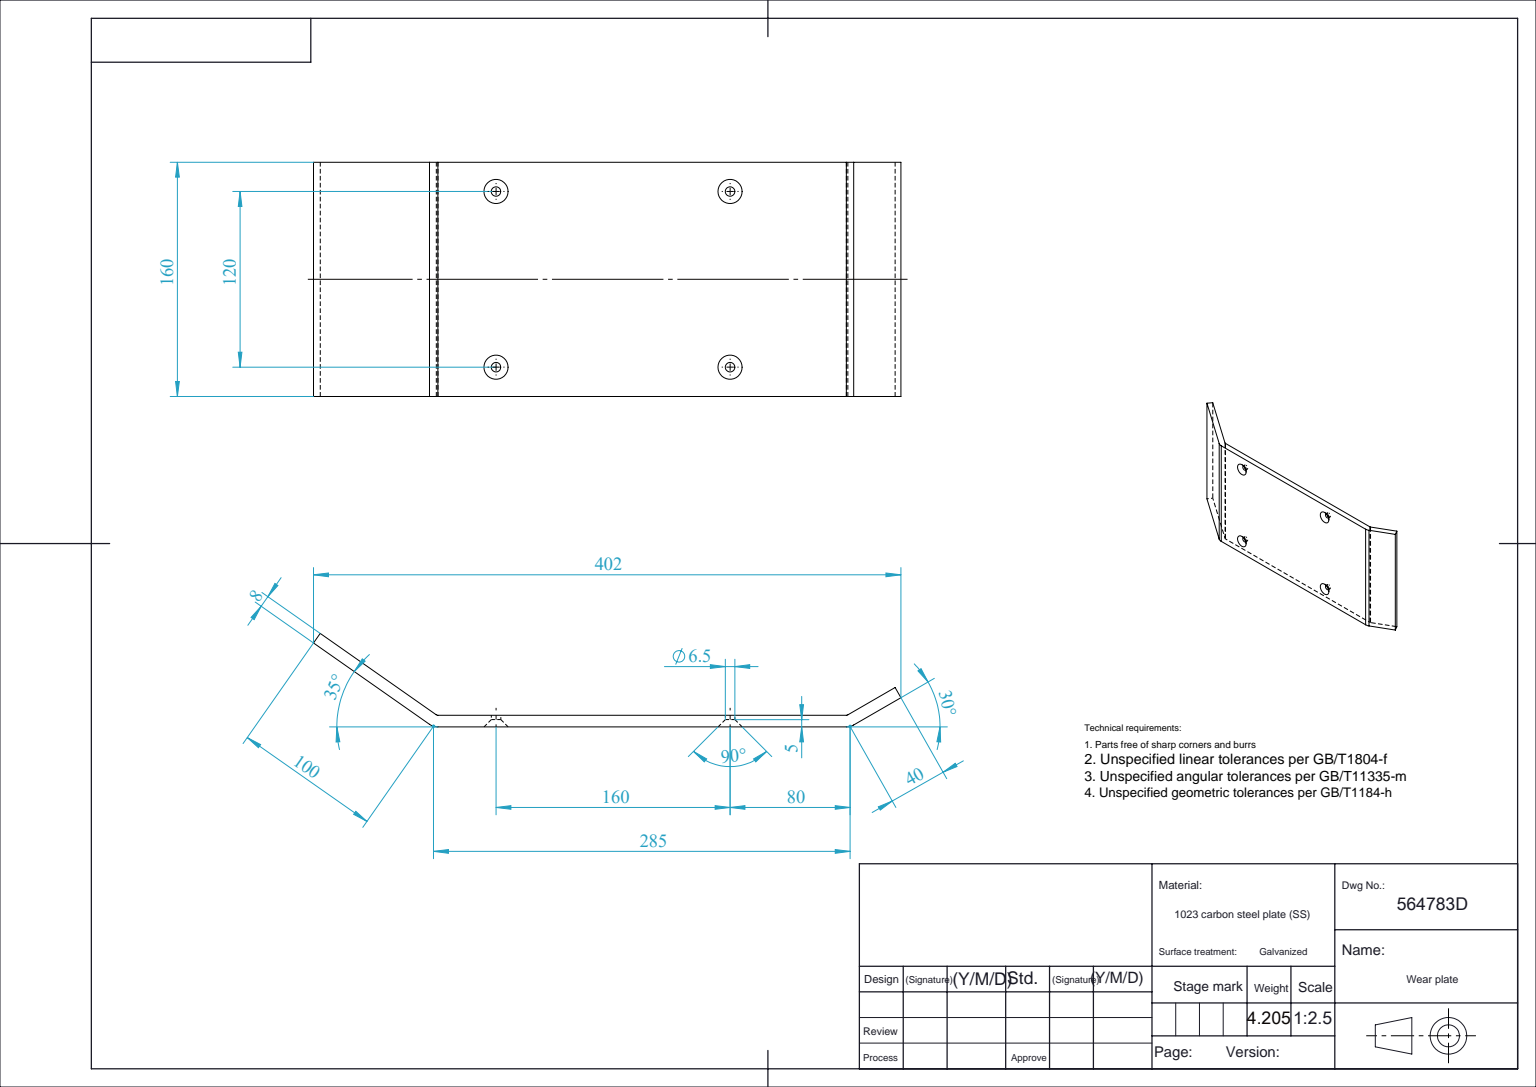
from build123d import *

# Parameters (mm, degrees)
BOSS_EXTRUDE4_DEPTH          = 160
SKETCH24_R                   = 3.25
CUT_EXTRUDE3_DEPTH           = 8
SKETCH26_R                   = 8.25
CUT_EXTRUDE4_DEPTH           = 5
CUT_EXTRUDE4_DRAFT           = -45
CUT_EXTRUDE4_PROFILE_2_DEPTH = 5
CUT_EXTRUDE4_PROFILE_2_DRAFT = -45
CUT_EXTRUDE4_PROFILE_3_DEPTH = 5
CUT_EXTRUDE4_PROFILE_3_DRAFT = -45
CUT_EXTRUDE4_PROFILE_4_DEPTH = 5
CUT_EXTRUDE4_PROFILE_4_DRAFT = -45
FILLET1_R                    = 10
FILLET2_R                    = 2


with BuildPart() as part:
    # Sketch23 → Boss-Extrude4 (new body)
    with BuildSketch(Plane.XY):
        Polygon((4.588611491, 6.553216354), (0, 0), (81.915204429, -57.357643635), (366.915204429, -57.357643635), (401.55622058, -37.357643635), (397.55622058, -30.429440405), (364.771610889, -49.357643635), (84.43759474, -49.357643635), align=None)
    extrude(amount=BOSS_EXTRUDE4_DEPTH)

    # Sketch24 → Cut-Extrude3 (cut)
    with BuildSketch(Plane(origin=(0, -49.357643635, 0), x_dir=(1, 0, 0), z_dir=(0, 1, 0))):
        with Locations(Location((124.771610889, -20, 0), (0, 0, 270))):
            Circle(SKETCH24_R)
        with Locations(Location((284.771610889, -20, 0), (0, 0, 270))):
            Circle(SKETCH24_R)
        with Locations(Location((124.771610889, -140, 0), (0, 0, 270))):
            Circle(SKETCH24_R)
        with Locations(Location((284.771610889, -140, 0), (0, 0, 270))):
            Circle(SKETCH24_R)
    extrude(amount=-CUT_EXTRUDE3_DEPTH, mode=Mode.SUBTRACT)


with BuildPart() as cut_extrude4_tool:
    # Sketch26 → Cut-Extrude4 (with draft: the straight prism first)
    with BuildSketch(Plane.XZ.offset(57.357643635)):
        with Locations((124.771610889, 140)):
            Circle(SKETCH26_R)
    extrude(amount=-CUT_EXTRUDE4_DEPTH)
    # Cut-Extrude4: the draft: its side faces are tilted about the plane it starts from
    cut_extrude4_sides = [cut_extrude4_tool.faces().sort_by_distance(p)[0] for p in [
        (116.521610889, -54.857643635, 140),
    ]]
    draft(cut_extrude4_sides, Plane.XZ.offset(57.357643635), CUT_EXTRUDE4_DRAFT)


with BuildPart() as part_1:
    add(part.part)

    # Cut-Extrude4: cut by cut_extrude4_tool
    add(cut_extrude4_tool.part, mode=Mode.SUBTRACT)


with BuildPart() as cut_extrude4_profile_2_tool:
    # Sketch26 → Cut-Extrude4 profile 2 (with draft: the straight prism first)
    with BuildSketch(Plane.XZ.offset(57.357643635)):
        with Locations((284.771610889, 140)):
            Circle(SKETCH26_R)
    extrude(amount=-CUT_EXTRUDE4_PROFILE_2_DEPTH)
    # Cut-Extrude4 profile 2: the draft: its side faces are tilted about the plane it starts from
    cut_extrude4_profile_2_sides = [cut_extrude4_profile_2_tool.faces().sort_by_distance(p)[0] for p in [
        (276.521610889, -54.857643635, 140),
    ]]
    draft(cut_extrude4_profile_2_sides, Plane.XZ.offset(57.357643635), CUT_EXTRUDE4_PROFILE_2_DRAFT)


with BuildPart() as part_2:
    add(part_1.part)

    # Cut-Extrude4 profile 2: cut by cut_extrude4_profile_2_tool
    add(cut_extrude4_profile_2_tool.part, mode=Mode.SUBTRACT)


with BuildPart() as cut_extrude4_profile_3_tool:
    # Sketch26 → Cut-Extrude4 profile 3 (with draft: the straight prism first)
    with BuildSketch(Plane.XZ.offset(57.357643635)):
        with Locations((284.771610889, 20)):
            Circle(SKETCH26_R)
    extrude(amount=-CUT_EXTRUDE4_PROFILE_3_DEPTH)
    # Cut-Extrude4 profile 3: the draft: its side faces are tilted about the plane it starts from
    cut_extrude4_profile_3_sides = [cut_extrude4_profile_3_tool.faces().sort_by_distance(p)[0] for p in [
        (276.521610889, -54.857643635, 20),
    ]]
    draft(cut_extrude4_profile_3_sides, Plane.XZ.offset(57.357643635), CUT_EXTRUDE4_PROFILE_3_DRAFT)


with BuildPart() as part_3:
    add(part_2.part)

    # Cut-Extrude4 profile 3: cut by cut_extrude4_profile_3_tool
    add(cut_extrude4_profile_3_tool.part, mode=Mode.SUBTRACT)


with BuildPart() as cut_extrude4_profile_4_tool:
    # Sketch26 → Cut-Extrude4 profile 4 (with draft: the straight prism first)
    with BuildSketch(Plane.XZ.offset(57.357643635)):
        with Locations((124.771610889, 20)):
            Circle(SKETCH26_R)
    extrude(amount=-CUT_EXTRUDE4_PROFILE_4_DEPTH)
    # Cut-Extrude4 profile 4: the draft: its side faces are tilted about the plane it starts from
    cut_extrude4_profile_4_sides = [cut_extrude4_profile_4_tool.faces().sort_by_distance(p)[0] for p in [
        (116.521610889, -54.857643635, 20),
    ]]
    draft(cut_extrude4_profile_4_sides, Plane.XZ.offset(57.357643635), CUT_EXTRUDE4_PROFILE_4_DRAFT)


with BuildPart() as part_4:
    add(part_3.part)

    # Cut-Extrude4 profile 4: cut by cut_extrude4_profile_4_tool
    add(cut_extrude4_profile_4_tool.part, mode=Mode.SUBTRACT)

    # Fillet1
    fillet1_edges = [part_4.edges().sort_by_distance(p)[0] for p in [
        (366.915204429, -57.357643635, 80),
        (81.915204429, -57.357643635, 80),
    ]]
    fillet(fillet1_edges, radius=FILLET1_R)

    # Fillet2
    fillet2_edges = [part_4.edges().sort_by_distance(p)[0] for p in [
        (84.43759474, -49.357643635, 80),
        (364.771610889, -49.357643635, 80),
    ]]
    fillet(fillet2_edges, radius=FILLET2_R)


solid = part_4.part
